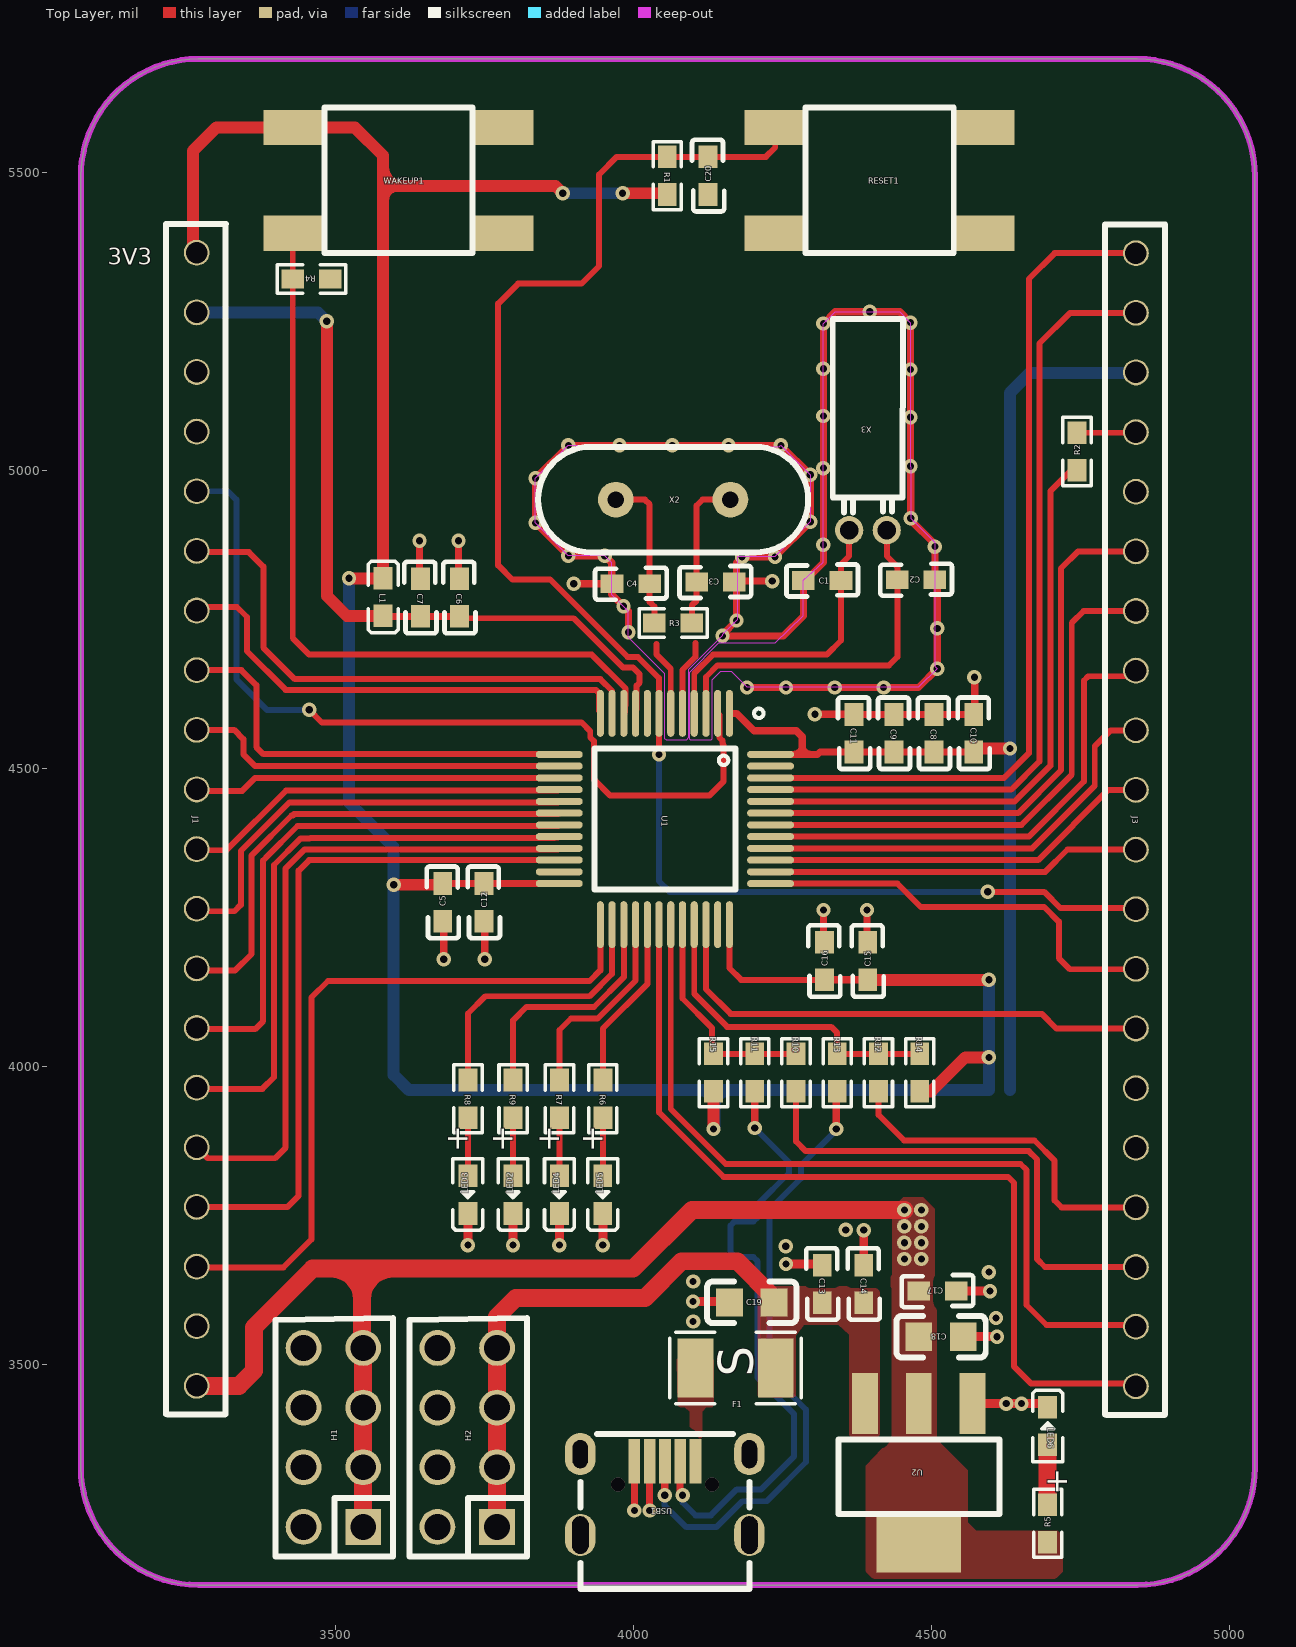
[diagram p0: Top Layer view]
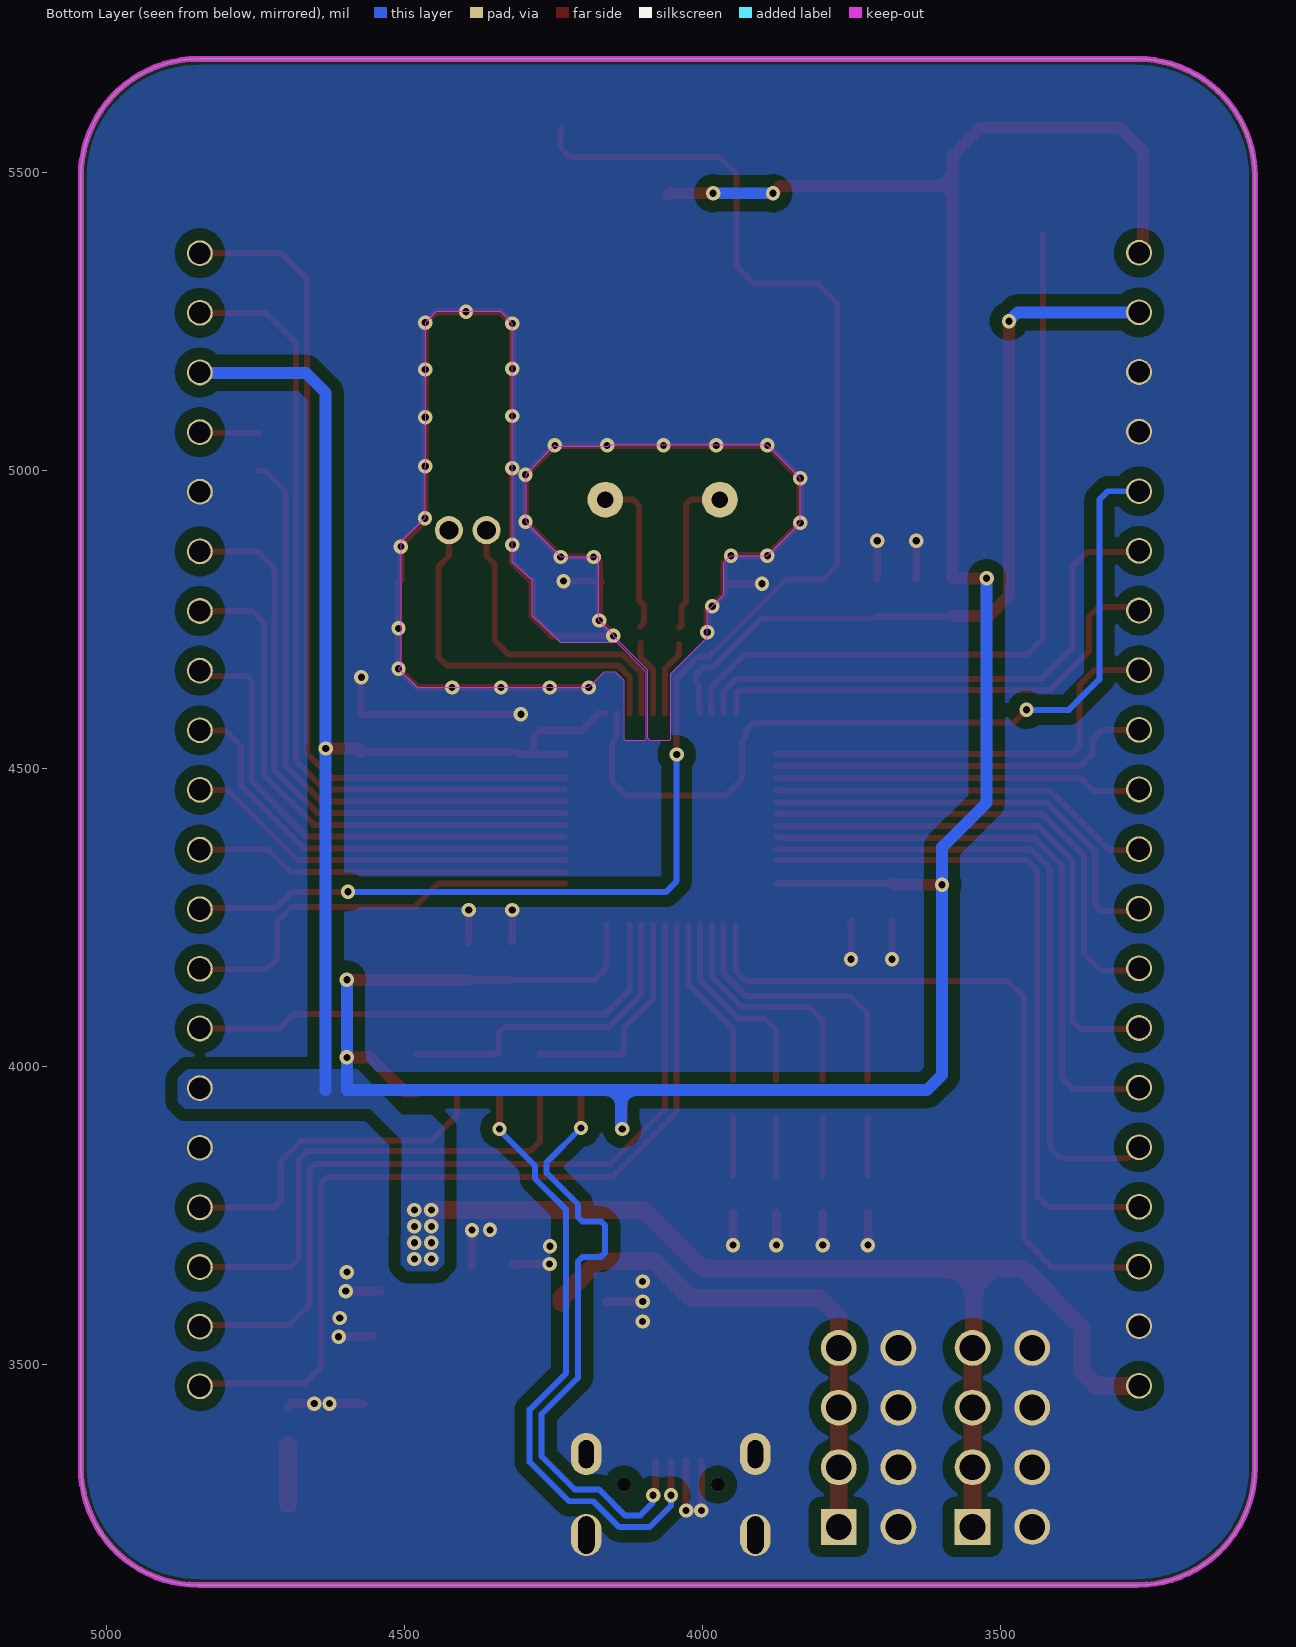
[diagram p1: Bottom Layer view, seen from below]
# Altium PCB MISC50188.pcbdoc
Units mil, origin at the board's own origin, x right, y up, seen from the top; angles counter-clockwise.
Board outline 1968.5 x 2559.06 mil, 2 copper layers (Top Layer, Bottom Layer), stack 62.206 mil thick; 53 components, 54 nets, 213 pads, 90 vias.

## Layer stack, top to bottom
Top Solder Mask Layer: solder mask 0.394, Dk 3.3
Top Layer: signal copper 1.379
Dielectric1: surface 59.449, FR4, Dk 4.5
Bottom Layer: signal copper 1.378
Bottom Solder Mask Layer: solder mask 0.394, Dk 3.3

## Board outline
3270.75,5689.88 ccw(c3270.75,5493.03) 3073.9,5493.03 3073.9,3327.68 ccw(c3270.75,3327.68) 3270.75,3130.83 4845.55,3130.83 ccw(c4845.55,3327.68) 5042.4,3327.68 5042.4,5493.03 ccw(c4845.55,5493.03) 4845.55,5689.88 3270.75,5689.88

## Design rules (kind name [scope] priority, off if disabled: settings)
BoardOutlineClearance copperThickness2oz_1 [All] p2 off: genericclearance=7.99 ignorepadtopadclearanceinfootprint=FALSE except(0: Arc-SplitContinuation Track-SplitContinuation SMDPad-SplitContinuation THPad-SplitContinuation Via-SplitContinuation Fill-SplitContinuation Region-SplitContinuation Poly-SplitContinuation Text-SplitContinuation Hole-SplitContinuation; 5.98: Arc-CutoutEdge Track-CutoutEdge SMDPad-CutoutEdge THPad-CutoutEdge Via-CutoutEdge Text-CutoutEdge; 6.9: Hole-OutlineEdge Hole-CutoutEdge; 11.81: Arc-OutlineEdge Track-OutlineEdge SMDPad-OutlineEdge THPad-OutlineEdge Via-OutlineEdge Fill-OutlineEdge Region-OutlineEdge Text-OutlineEdge Fill-CutoutEdge Region-CutoutEdge; 20: Poly-OutlineEdge Poly-CutoutEdge)
BoardOutlineClearance Plane_innerPlane_1 [All] p4 off: genericclearance=8 ignorepadtopadclearanceinfootprint=FALSE except(0: Arc-SplitContinuation Track-SplitContinuation SMDPad-SplitContinuation THPad-SplitContinuation Via-SplitContinuation Fill-SplitContinuation Region-SplitContinuation Poly-SplitContinuation Text-SplitContinuation Hole-SplitContinuation; 5.98: Arc-CutoutEdge Track-CutoutEdge SMDPad-CutoutEdge THPad-CutoutEdge Via-CutoutEdge Text-CutoutEdge; 6.9: Hole-OutlineEdge Hole-CutoutEdge; 10: Poly-OutlineEdge Poly-CutoutEdge; 11.81: Arc-OutlineEdge Track-OutlineEdge SMDPad-OutlineEdge THPad-OutlineEdge Via-OutlineEdge Fill-OutlineEdge Region-OutlineEdge Text-OutlineEdge Fill-CutoutEdge Region-CutoutEdge)
BoardOutlineClearance Copper_copperRegion_1 [All] p6 off: genericclearance=8 ignorepadtopadclearanceinfootprint=FALSE except(0: Arc-SplitContinuation Track-SplitContinuation SMDPad-SplitContinuation THPad-SplitContinuation Via-SplitContinuation Fill-SplitContinuation Region-SplitContinuation Poly-SplitContinuation Text-SplitContinuation Hole-SplitContinuation; 5.98: Arc-CutoutEdge Track-CutoutEdge SMDPad-CutoutEdge THPad-CutoutEdge Via-CutoutEdge Text-CutoutEdge; 6.9: Hole-OutlineEdge Hole-CutoutEdge; 10: Poly-OutlineEdge Poly-CutoutEdge; 11.81: Arc-OutlineEdge Track-OutlineEdge SMDPad-OutlineEdge THPad-OutlineEdge Via-OutlineEdge Fill-OutlineEdge Region-OutlineEdge Text-OutlineEdge Fill-CutoutEdge Region-CutoutEdge)
BoardOutlineClearance copperThickness1oz_1 [All] p8: genericclearance=8 ignorepadtopadclearanceinfootprint=FALSE except(0: Arc-SplitContinuation Track-SplitContinuation SMDPad-SplitContinuation THPad-SplitContinuation Via-SplitContinuation Fill-SplitContinuation Region-SplitContinuation Poly-SplitContinuation Text-SplitContinuation Hole-SplitContinuation; 5.98: Arc-CutoutEdge Track-CutoutEdge SMDPad-CutoutEdge THPad-CutoutEdge Via-CutoutEdge Text-CutoutEdge; 6.9: Hole-OutlineEdge Hole-CutoutEdge; 11.81: Arc-OutlineEdge Track-OutlineEdge SMDPad-OutlineEdge THPad-OutlineEdge Via-OutlineEdge Fill-OutlineEdge Region-OutlineEdge Text-OutlineEdge Fill-CutoutEdge Region-CutoutEdge; 20: Poly-OutlineEdge Poly-CutoutEdge)
Clearance copperThickness2oz [All] p1 off: gap=7.99 ignorepadtopadclearanceinfootprint=FALSE except(5.98: SMDPad-Track SMDPad-SMDPad THPad-Track SMDPad-THPad THPad-THPad Track-Via SMDPad-Via THPad-Via Via-Via Fill-SMDPad Region-SMDPad Fill-THPad Region-THPad Fill-Via Region-Via Fill-Fill Fill-Region Region-Region Arc-Track Arc-SMDPad Arc-THPad Arc-Via Fill-Arc Region-Arc Arc-Arc Text-Track SMDPad-Text Text-THPad Text-Via Fill-Text Region-Text Arc-Text Text-Text; 6.9: Hole-Track Hole-SMDPad Hole-THPad Hole-Via Fill-Hole Region-Hole Hole-Arc Hole-Text; 11.81: Fill-Track Region-Track; 20: Poly-Track Poly-SMDPad Poly-THPad Poly-Via Poly-Fill Poly-Region Poly-Poly Poly-Arc Poly-Text Poly-Hole)
Clearance Plane_innerPlane [All] p3 off: gap=8 ignorepadtopadclearanceinfootprint=FALSE except(5.98: SMDPad-Track SMDPad-SMDPad THPad-Track SMDPad-THPad THPad-THPad Track-Via SMDPad-Via THPad-Via Via-Via Fill-SMDPad Region-SMDPad Fill-THPad Region-THPad Fill-Via Region-Via Fill-Fill Fill-Region Region-Region Arc-Track Arc-SMDPad Arc-THPad Arc-Via Fill-Arc Region-Arc Arc-Arc Text-Track SMDPad-Text Text-THPad Text-Via Fill-Text Region-Text Arc-Text Text-Text; 6.9: Hole-Track Hole-SMDPad Hole-THPad Hole-Via Fill-Hole Region-Hole Hole-Arc Hole-Text; 10: Poly-Track Poly-SMDPad Poly-THPad Poly-Via Poly-Fill Poly-Region Poly-Poly Poly-Arc Poly-Text Poly-Hole; 11.81: Fill-Track Region-Track)
Clearance Copper_copperRegion [All] p5 off: gap=8 ignorepadtopadclearanceinfootprint=FALSE except(5.98: SMDPad-Track SMDPad-SMDPad THPad-Track SMDPad-THPad THPad-THPad Track-Via SMDPad-Via THPad-Via Via-Via Fill-SMDPad Region-SMDPad Fill-THPad Region-THPad Fill-Via Region-Via Fill-Fill Fill-Region Region-Region Arc-Track Arc-SMDPad Arc-THPad Arc-Via Fill-Arc Region-Arc Arc-Arc Text-Track SMDPad-Text Text-THPad Text-Via Fill-Text Region-Text Arc-Text Text-Text; 6.9: Hole-Track Hole-SMDPad Hole-THPad Hole-Via Fill-Hole Region-Hole Hole-Arc Hole-Text; 11.81: Fill-Track Region-Track; 20: Poly-Track Poly-SMDPad Poly-THPad Poly-Via Poly-Fill Poly-Region Poly-Poly Poly-Arc Poly-Text Poly-Hole)
Clearance copperThickness1oz [All] p7: gap=8 ignorepadtopadclearanceinfootprint=FALSE except(5.98: SMDPad-Track SMDPad-SMDPad THPad-Track SMDPad-THPad THPad-THPad Track-Via SMDPad-Via THPad-Via Via-Via Fill-SMDPad Region-SMDPad Fill-THPad Region-THPad Fill-Via Region-Via Fill-Fill Fill-Region Region-Region Arc-Track Arc-SMDPad Arc-THPad Arc-Via Fill-Arc Region-Arc Arc-Arc Text-Track SMDPad-Text Text-THPad Text-Via Fill-Text Region-Text Arc-Text Text-Text; 6.9: Hole-Track Hole-SMDPad Hole-THPad Hole-Via Fill-Hole Region-Hole Hole-Arc Hole-Text; 11.81: Fill-Track Region-Track; 20: Poly-Track Poly-SMDPad Poly-THPad Poly-Via Poly-Fill Poly-Region Poly-Poly Poly-Arc Poly-Text Poly-Hole)
DiffPairsRouting differentialPair [All] p1: maxlimit=6 minlimit=6 mostfreqgap=6 toplayer_minwidth=5 toplayer_prefwidth=10 toplayer_maxwidth=100 toplayer_mingap=6 toplayer_prefgap=6 toplayer_maxgap=6 bottomlayer_minwidth=5 bottomlayer_prefwidth=10 bottomlayer_maxwidth=100 bottomlayer_mingap=6 bottomlayer_prefgap=6 bottomlayer_maxgap=6 maxuncoupledlength=10
HoleToHoleClearance otherClearance [All] p1: gap=11.81 allowstackedmicrovias=TRUE
Length netLength [All] p1: minlimit=0 maxlimit=0
PasteMaskExpansion pasteMaskExpansion [All] p1: expansion=0
PlaneConnect innerPlane [All] p1: planeconnectstyle=Relief reliefexpansion=20 reliefentries=4 reliefconductorwidth=10 reliefairgap=10
PolygonConnect copperRegion [All] p1: connectstyle=Direct reliefconductorwidth=10 reliefentries=4 polygonreliefangle="90 Angle" airgapwidth=10 via.connectstyle=Relief via.reliefconductorwidth=10 via.reliefentries=4 via.polygonreliefangle="90 Angle" via.airgapwidth=10
RoutingVias viaSize [All] p1: holewidth=12.01 width=24.02 viastyle="Through Hole" minholewidth=11.81 minwidth=19.68 maxholewidth=248.03 maxwidth=393.7
SolderMaskExpansion solderMaskExpansion [IsVia] p1: expansion=-1000 istentingtop=TRUE
SolderMaskExpansion solderMaskExpansion [All] p2: expansion=2 istentingtop=FALSE
Width copperThickness2oz_2 [All] p1 off: maxlimit=100 minlimit=8 preferedwidth=10
Width power [(InNet('GND') OR InNet('VCC_3V3') OR InNet('VDDA') OR InNet('VIN_5V'))] p2: maxlimit=100 minlimit=10 preferedwidth=30
Width copperThickness1oz_2 [All] p3: maxlimit=100 minlimit=5 preferedwidth=10

## Components (designator, comment, footprint, x,y, rotation, side; value= is the part's Value field where it differs from the comment)
C1 "20pF" C0603 4316.93,3045.28 r0 top
C2 "20pF" C0603 4474.41,6586.61 r180 top
C3 "20pF" C0603 4137.8,6582.68 r180 top
C4 "20pF" C0603 3996.06,3039.93 r0 top
C5 "1uF" C0603 5450.78,4275.59 r90 top
C6 "10nF" C0603 1938.58,4786.54 r270 top
C7 "1uF" C0603 1873.2,4786.54 r270 top
C8 "1uF" C0603 2734.25,4559.06 r270 top
C9 "10nF" C0603 2667.32,4559.06 r270 top
C10 "1uF" C0603 2801.18,4559.06 r270 top
C11 "10nF" C0603 2600.39,4559.06 r270 top
C12 "10nF" C0603 5519.68,4275.59 r90 top
C13 "1uF" C0603 2546.93,3635.83 r270 top
C14 "10nF" C0603 2616.61,3635.83 r270 top
C15 "1uF" C0603 6163.38,4177.17 r90 top
C16 "10nF" C0603 6090.55,4177.17 r90 top
C17 "100nf" C0603 4510.24,5393.7 r180 top
C18 "10uf" C0805 4516.14,3547.25 r180 top
C19 "22uF" C0805 4198.9,3604.88 r0 top
C20 "100nF" C0603 5895.66,5494.09 r90 top
F1 "" F1210 4171.65,3494.88 r0 top
H1 "" HDR-TH_8P-P2.54-V-M-R2-C4-S2.54 3547.24,3228.35 r90 top
H2 "" HDR-TH_8P-P2.54-V-M-R2-C4-S2.54 3771.65,3228.35 r90 top
J1 "" HDR-TH_20PIN-V-MALE-PITCH2.54 3268.11,5364.88 r270 top
J3 "" HDR-TH_20PIN-V-MALE-PITCH2.54 4842.91,5364.09 r270 top
L1 "3.3uH" L0603 3580.71,4787.53 r270 top
LED2 "" LED0603 3798.42,3785.44 r90 top
LED3 "" LED0603 3722.83,3785.44 r90 top
LED4 "" LED0603 3876.27,3785.44 r90 top
LED5 "" LED0603 3949,3785.44 r90 top
LED6 "" LED0603 4694.88,3397.64 r270 top
R1 "10K" R0603 4057.08,5494.09 r270 top
R2 "10K" R0603 4744.09,5031.5 r90 top
R3 "1M" R0603 4066.93,4744.1 r0 top
R4 "10K" R0603 3460.63,5320.87 r180 top
R5 "1K" R0603 4694.88,3234.25 r90 top
R6 "1K" R0603 3949.2,3946.09 r270 top
R7 "1K" R0603 3876.47,3946.09 r270 top
R8 "1K" R0603 3723.03,3946.09 r270 top
R9 "1K" R0603 3798.62,3946.09 r270 top
R10 "0R" R0603 4272.94,3990.16 r270 top
R11 "NC/22R" R0603 4203.81,3990.16 r270 top
R12 "0R" R0603 4411.19,3990.16 r270 top
R13 "NC/22R" R0603 4342.06,3990.16 r270 top
R14 "NC/1.5K" R0603 4480.31,3990.16 r270 top
R15 "NC/1.5K" R0603 4134.69,3990.16 r270 top
RESET1 "" SW-SMD-T6X6-9.5X5.8 4413.38,5486.22 r0 top
U1 "" TQFP-48_L7.0-W7.0-P0.50-LS9.0-BL 4053.15,4415.35 r180 top
U2 "" SOT-223 4568.9,3435.04 r180 top
USB1 "" U-F-M5DD-Y-1 4053.15,3214.57 r180 top
WAKEUP1 "" SW-SMD-T6X6-9.5X5.8 3606.3,5486.22 r0 top
X2 "8MHz" OSC-49S-1 4066.93,4950.79 r0 top
X3 "32.768kHz" DT-38_BD3.1-P0.80 4393.7,4899.61 r180 top

## Footprints (in the part's own frame and the unit in brackets; to place one, negate y for a bottom-side part, rotate by r counter-clockwise, add the part's x,y. Pads: shape width x height; smd on the part's side, far side on the other; paste and mask are expansions set on the pad)
C0603 [mm]
  rect 0.965x0.8 smd: 1(-0.8,44.958) 2(0.8,44.958)
  silkscreen extent -1.52,44.27 1.52,45.64
C0805 [mm]
  rect 1.14x1.2 smd: 1(-0.95,0) 2(0.95,0)
  silkscreen extent -1.91,-0.89 1.91,0.89
DT-38_BD3.1-P0.80 [mm]
  round 1.2 hole 0.8: 1(-0.8,0) 2(0.8,0)
  silkscreen extent -1.5,-9 1.5,-0.76
F1210 [mm]
  rect 1.52x2.5 smd: 1(-1.71,0) 2(1.71,0)
  silkscreen extent -2.79,-1.52 2.79,1.52
HDR-TH_8P-P2.54-V-M-R2-C4-S2.54 [mil]
  rect 60x60 hole 43.31: 1(0,0)
  round 60 hole 43.31: 2(0,100) 3(100,0) 4(100,100) 5(200,0) 6(200,100) 7(300,0) 8(300,100)
  silkscreen extent -50,-50 350,147
HDR-TH_20PIN-V-MALE-PITCH2.54 [mm]
  round 1.1 hole 0.914: 1(0,0) 2(2.54,0) 3(5.08,0) 4(7.62,0) 5(10.16,0) 6(12.7,0) 7(15.24,0) 8(17.78,0) 9(20.32,0) 10(22.86,0) 11(25.4,0) 12(27.94,0) 13(30.48,0) 14(33.02,0) 15(35.56,0) 16(38.1,0) 17(40.64,0) 18(43.18,0) 19(45.72,0) 20(48.26,0)
  silkscreen extent -1.23,-1.31 49.49,1.25
L0603 [mm]
  rect 0.965x0.8 smd: 1(-0.8,0) 2(0.8,0)
  silkscreen extent -1.52,-0.64 1.52,0.64
LED0603 [mm]
  rect 0.965x0.8 smd: 1(-0.8,0) 2(0.8,0)
  silkscreen extent -1.52,-0.64 1.52,0.64
OSC-49S-1 [mil]
  round 60 hole 27.56: 1(-96.06,0) 2(96.06,0)
  silkscreen extent -226,-89 226,89
R0603 [mm]
  rect 0.965x0.8 smd: 1(-0.8,0) 2(0.8,0)
  silkscreen extent -1.45,-0.6 1.45,0.6
SOT-223 [mm]
  rect 1.1x2.6 smd: 1(0,0) 2(2.29,0) 3(4.58,0)
  rect 3.6x2.4 smd: 4(2.29,6)
  silkscreen extent -1.14,1.52 5.71,4.7
SW-SMD-T6X6-9.5X5.8 [mm]
  rect 2.5x1.5 smd: 1(-4.5,2.25) 2(4.5,2.25) 3(-4.5,-2.25) 4(4.5,-2.25)
  silkscreen extent -3.15,-3.1 3.15,3.1
TQFP-48_L7.0-W7.0-P0.50-LS9.0-BL [mm]
  oval 0.3x2 smd: 1(-2.75,-4.5) 2(-2.25,-4.5) 3(-1.75,-4.5) 4(-1.25,-4.5) 5(-0.75,-4.5) 6(-0.25,-4.5) 7(0.25,-4.5) 8(0.75,-4.5) 9(1.25,-4.5) 10(1.75,-4.5) 11(2.25,-4.5) 12(2.75,-4.5) 25(2.75,4.5) 26(2.25,4.5) 27(1.75,4.5) 28(1.25,4.5) 29(0.75,4.5) 30(0.25,4.5) 31(-0.25,4.5) 32(-0.75,4.5) 33(-1.25,4.5) 34(-1.75,4.5) 35(-2.25,4.5) 36(-2.75,4.5)
  oval 2x0.3 smd: 13(4.5,-2.75) 14(4.5,-2.25) 15(4.5,-1.75) 16(4.5,-1.25) 17(4.5,-0.75) 18(4.5,-0.25) 19(4.5,0.25) 20(4.5,0.75) 21(4.5,1.25) 22(4.5,1.75) 23(4.5,2.25) 24(4.5,2.75) 37(-4.5,2.75) 38(-4.5,2.25) 39(-4.5,1.75) 40(-4.5,1.25) 41(-4.5,0.75) 42(-4.5,0.25) 43(-4.5,-0.25) 44(-4.5,-0.75) 45(-4.5,-1.25) 46(-4.5,-1.75) 47(-4.5,-2.25) 48(-4.5,-2.75)
  silkscreen extent -4.2,-4.7 3,3
U-F-M5DD-Y-1 [mm]
  rect 0.5x1.9 smd: 1(-1.3,-3.15) 2(-0.65,-3.15) 3(0,-3.15) 4(0.65,-3.15) 5(1.3,-3.15)
  oval 1.3x1.8 hole 0.65 slot 1.2 at 90 deg: 6(-3.6,-3.45) 7(3.6,-3.45)
  oval 1.3x1.8 hole 0.7 slot 1.6 at 90 deg: 8(3.6,0) 9(-3.6,0)
  silkscreen extent -3.6,-4.3 3.6,2.3

## Via types
v1: diameter 24.02, hole 12, Top Layer to Bottom Layer, 88 vias
v2: diameter 23.62, hole 23.6, Top Layer to Bottom Layer, 2 vias

## Nets (pads, with @x,y where several pads share a name; then routed paths per layer and width w, separated by ;. In a path a pad name is that pad's centre, name@x,y a point inside that pad or via, vN(x,y) a via of type N, cw(c..) or ccw(c..) an arc to the next point about the centre after c; other vN are vias at no path point)
$1N278: LED5.2 R6.2 | length 97.7
  Top Layer w10: LED5.2 3949.2,3817.13 R6.2
$1N354: LED4.2 R7.2 | length 97.7
  Top Layer w10: LED4.2 3876.47,3817.13 R7.2
$1N427: LED3.2 R8.2 | length 97.7
  Top Layer w10: LED3.2 3723.03,3817.13 R8.2
$1N500: LED2.2 R9.2 | length 97.7
  Top Layer w10: LED2.2 3798.62,3817.13 R9.2
$1N3002: LED6.2 R5.2 | length 100.4
  Top Layer w30: R5.2 LED6.2
$1N3542: F1.1 USB1.1
$1N7842: J3.4 R2.2 | length 99.3
  Top Layer w10: R2.2 4841.81,5062.99 J3.4
$1N14164: R12.1 R13.1 R14.1 U1.33 | length 556.3
  Top Layer w10: U1.33 4102.36,4122.05 4157.48,4066.93 4332.06,4066.93 4342.06,4056.93 R13.1 R12.1 R14.1
$1N14239: R10.1 R11.1 R15.1 U1.32 | length 377.5
  Top Layer w10: U1.32 4082.68,4114.31 4131.89,4065.1 4131.89,4022.49 4132.72,4021.66 R15.1 R11.1 R10.1
BOOT0: R2.1 U1.44 | length 1013.5
  Top Layer w10: U1.44 4639.62,4444.88 4699.38,4504.64 4699.38,4965.14 4734.25,5000 R2.1
D+: R13.2 USB1.3 | length 1065.7
  Top Layer w12: v1(4052.86,3281.5) 4052.86,3338.3 USB1.3 ; v1(4340.55,3895.67) 4340.55,3957.15 R13.2
  Bottom Layer w10: v1(4052.86,3281.5) 4052.86,3263.99 4089,3227.86 4139.55,3227.86 4183.07,3271.37 4223.99,3271.37 4289.86,3337.25 4289.86,3424.99 4228.63,3486.22 4228.63,3759.93 4281.18,3812.48 4281.18,3834.34 4340.55,3893.7 v1(4340.55,3895.67)
D-: R11.2 USB1.2 | length 1065.3
  Top Layer w12: USB1.2 4078.74,3285.62 v1(4082.86,3281.5) ; v1(4203.81,3897.19) R11.2
  Bottom Layer w10: v1(4082.86,3281.5) 4082.77,3281.41 4082.77,3269.39 4104.42,3247.73 4130.22,3247.73 4173.74,3291.25 4214.66,3291.25 4269.99,3346.58 4269.99,3417.44 4208.75,3478.68 4208.75,3673.65 4201.68,3680.72 4170.45,3680.72 4163.38,3687.79 4163.38,3733.65 4170.45,3740.72 4201.68,3740.72 4208.75,3747.79 4208.75,3769.26 4261.31,3821.81 4261.31,3839.69 v1(4203.81,3897.19)
GND: C1.1 C2.1 C3.1 C4.1 C5.1 C6.1 C7.1 C8.1 C9.1 C10.1 C11.1 C12.1 C13.1 C14.1 C15.2 C16.2 C17.1 C18.1 C19.1 C20.1 H1.2 H1.4 H1.6 H1.8 H2.2 H2.4 H2.6 H2.8 J1.3 J1.4 J1.19 J3.5 J3.16 LED2.1 LED3.1 LED4.1 LED5.1 LED6.1 R4.1 RESET1.3 U1.8 U1.23 U1.35 U1.47 U2.1 USB1.4 USB1.5 USB1.6 USB1.7 USB1.8 USB1.9 | length 4596.1
  Top Layer w12: v1(3641.73,4881.89) 3641.73,4819.51 C7.1 ; C5.1 3682.26,4242.62 v1(3682.26,4180.25) ; v1(3707.11,4881.89) 3707.11,4819.51 C6.1 ; C12.1 3751.15,4242.62 v1(3751.15,4180.25) ; v1(3900.29,4809.9) 3962.66,4809.9 C4.1@3964.14,4811.38 ; v1(3992.12,4728.45) 3992.12,4763.78 v1(3983.83,4772.08) 3964.14,4791.77 C4.1@3964.14,4811.38 ; v1(4001.97,3255.91) USB1.5 ; v1(4027.56,3255.91) USB1.4 ; v1(4149.6,4722.44) 4251.97,4722.44 4285.43,4755.91 C1.1 4288.68,4815.28 4318.9,4845.5 v1(4318.9,4875.25) v1(4318.9,5003.71) v1(4318.9,5091.06) v1(4318.9,5170.19) v1(4318.9,5246.06) 4338.58,5265.75 v1(4396.62,5265.75) 4446.85,5265.75 v1(4464.94,5247.65) v1(4464.94,5169.12) v1(4464.9,5089) ; v1@4149.6,4724.41 v1(4173.23,4748.04) C3.1@4173.23,4814.15 ; C3.1 4170.77,4814.15 C3.1@4173.23,4814.15 ; v1(4190.94,4635.83) v1(4256.11,4635.83) v1(4337.97,4635.83) v1(4419.92,4635.83) 4478.34,4635.83 v1(4509.84,4667.32) v1(4509.84,4734.91) 4509.84,4812.68 C2.1 v1(4505.9,4872.05) ; v1(4233.14,4814.15) C3.1@4173.23,4814.15 ; v1(4304.58,4591.05) 4369.9,4591.05 C11.1 C9.1 C8.1 C10.1 ; v1(4319.07,4262.67) 4319.07,4210.14 C16.2 ; v1(4391.91,4262.67) 4391.91,4210.14 C15.2 ; v1(4464.9,5089) v1(4464.9,5006.79) 4465.45,5006.24 v1(4465.45,4919.5) ; v1@4465.45,4916.44 v1@4505.9,4875.99 ; C10.1@4571.18,4592.03 4572.64,4590.57 4572.64,4652.45 v1(4572.04,4653.05) ; C4.1@3964.14,4811.38 3964.14,4844.92 v1(3952.33,4856.73) v1(3891.3,4856.73) v1(3836.18,4911.85) v1(3836.18,4986.65) v1(3891.3,5041.77) v1(3977.03,5041.77) v1(4065.49,5041.77) v1(4159.94,5041.77) v1(4247.6,5041.77) v1(4296.81,4992.56) v1(4296.81,4913.82) v1(4237.76,4854.76) v1(4182.64,4854.76) 4173.23,4845.35 C3.1@4173.23,4814.15
  Top Layer w15: v1(3722.83,3700.79) LED3.1 ; v1(3798.42,3700.79) LED2.1 ; v1(3876.27,3700.79) LED4.1 ; v1(3949,3700.79) LED5.1 ; v1(4100.39,3606.3) 4160.07,3606.3 C19.1 ; v1(4256.37,3669.29) 4314.96,3669.29 C13.1 C13.1@4317.48,3667.87 ; v1(4386.61,3725.92) C14.1 C14.1@4387.16,3666.78 ; C17.1@4541.19,3623.15 C17.1 v1(4598.35,3623.7) ; C18.1 v1(4610.16,3547.25) ; U2.1 v1(4625.52,3435.04) v1(4651.16,3435.04) 4688.98,3435.04 LED6.1
  other v1: 4100.5,3572.83 4608.26,3578.74 4100.5,3639.88 4596.45,3655.52 4255.9,3698.82 4356.3,3726.38
NRST: C20.2 J3.12 R1.1 RESET1.1 U1.7 | length 2643.8
  Top Layer w10: v1(4043.3,4523.62) U1.7 4043.31,4651.57 4007.87,4687.01 3990.66,4687.01 3860.74,4816.93 3797.24,4816.93 3773.62,4840.55 3773.62,5279.53 3807.09,5312.99 3913.38,5312.99 3942.91,5342.52 3942.91,5496.06 3972.44,5525.59 R1.1 C20.2 4222.44,5525.59 4238.19,5541.34 4238.19,5572.83 RESET1.1 ; v1(4594.48,4293.31) 4688.97,4293.31 4716.53,4265.75 4841.26,4265.75 J3.12
  Bottom Layer w10: v1(4043.3,4523.62) 4043.3,4311.03 4061.02,4293.31 v1(4594.48,4293.31)
OSC32IN: C2.2 U1.3 X3.1 | length 615.7
  Top Layer w10: U1.3 4122.05,4653.55 4141.45,4672.95 4428.85,4672.95 4442.91,4687.01 C2.2 4442.91,4838.58 4425.19,4856.3 X3.1
OSC32OUT: C1.2 U1.4 X3.2 | length 526.6
  Top Layer w10: U1.4 4102.36,4659.45 4133.86,4690.95 4324.8,4690.95 4348.42,4714.57 C1.2 4348.42,4842.52 4362.2,4856.3 X3.2
OSC_IN: C3.2 R3.2 U1.5 X2.2 | length 396.3
  Top Layer w10: U1.5 4082.68,4665.36 4104.33,4687.01 4104.33,4710.63 ; R3.2@4104.33,4738.19 R3.2 4098.43,4773.63 4106.3,4781.5 C3.2 4106.3,4940.95 4116.14,4950.79 X2.2
OSC_OUT: C4.2 R3.1 U1.6 X2.1 | length 397.5
  Top Layer w10: X2.1 4019.68,4950.79 4027.56,4942.91 C4.2 4027.56,4779.53 4035.43,4771.65 R3.1 4035.43,4740.16 R3.1@4039.37,4736.22 ; 4039.37,4708.67 4039.37,4690.95 4062.99,4667.32 U1.6
PA0/WAKEUP: R4.2 U1.10 WAKEUP1.3 | length 1312.9
  Top Layer w10: WAKEUP1.3@3429.13,5395.67 R4.2 3429.13,4718.51 3456.69,4690.95 3930.49,4690.95 3987.05,4634.39 3987.05,4606 3985.94,4604.89 3985.94,4594.2 U1.10
PA1: J1.6 U1.11 | length 910.9
  Top Layer w10: J1.6 3270.08,4862.91 3355.59,4862.91 3379.92,4838.58 3379.92,4702.76 3432.79,4649.89 3944.86,4649.89 3964.57,4630.19 U1.11
PA2: J1.7 U1.12 | length 805.2
  Top Layer w10: J1.7 3274.02,4770.79 3335.51,4770.79 3352.36,4753.94 3352.36,4696.85 3417.32,4631.89 3937.41,4631.89 3942.91,4626.38 3942.91,4596.82 3944.34,4595.39 3944.34,4593.06 U1.12
PA3: J1.8 U1.13 | length 727.3
  Top Layer w10: J1.8 3342.99,4664.88 3368.11,4639.77 3368.11,4535.84 3379.92,4524.03 3875.58,4524.03 U1.13
PA4: J1.9 U1.14 | length 648.1
  Top Layer w10: J1.9 3330.79,4564.88 3346.46,4549.21 3346.46,4523.62 3366.14,4503.94 U1.14
PA5: J1.10 U1.15 | length 617.8
  Top Layer w10: J1.10 3270.39,4462.6 3344.49,4462.6 3366.14,4484.25 U1.15
PA6: J1.11 U1.16 | length 650.8
  Top Layer w10: J1.11 3270.08,4362.91 3317.9,4362.91 3417.87,4462.88 3874.3,4462.88 U1.16
PA7: J1.12 U1.17 | length 738.9
  Top Layer w10: J1.12 3270.08,4264.88 3274.31,4260.65 3331.51,4260.65 3342.24,4271.37 3342.24,4361.79 3423.36,4442.91 3868.24,4442.91 3868.53,4443.2 3874.3,4443.2 U1.17
PA8: R6.1 U1.29 | length 291.4
  Top Layer w10: R6.1 3949.2,4064.07 4023.62,4138.49 U1.29
PA9: J3.20 U1.30 | length 1485
  Top Layer w10: U1.30 4043.31,3923.36 4151.71,3814.96 4628.78,3814.96 4638.78,3804.96 4638.78,3497.05 4667.32,3468.51 4838.5,3468.51 J3.20
PA10: J3.19 U1.31 | length 1372.9
  Top Layer w10: U1.31 4062.99,3929.14 4155.23,3836.9 4649.45,3836.9 4659.45,3826.9 4659.45,3600.4 4692.91,3566.93 4840.07,3566.93 J3.19
PA11: J3.18 R10.2 | length 839.1
  Top Layer w10: R10.2 4272.94,3874.7 4289.37,3858.27 4663.53,3858.27 4677.45,3844.36 4677.45,3677.17 4690.52,3664.09 J3.18
PA12: J3.17 R12.2 | length 574.5
  Top Layer w10: R12.2 4411.41,3958.44 4411.41,3919.29 4454.44,3876.27 4672.94,3876.27 4706.69,3842.52 4706.69,3775.59 4718.19,3764.09 J3.17
PA15: J3.11 U1.38 | length 628.1
  Top Layer w10: U1.38 4690.94,4326.77 4728.26,4364.09 J3.11
PB0: J1.13 U1.18 | length 815.4
  Top Layer w10: J1.13 3271.57,4161.42 3332.68,4161.42 3360.24,4188.98 3360.24,4354.33 3427.16,4421.26 3429.27,4421.26 3431.52,4423.51 3874.3,4423.51 U1.18
PB1: J1.14 U1.19 | length 908.6
  Top Layer w10: J1.14 3270.08,4062.91 3366.06,4062.91 3379.64,4076.49 3379.64,4345.77 3383.86,4349.99 3383.86,4350.4 3437,4403.54 3868.24,4403.54 3868.53,4403.83 3874.3,4403.83 U1.19
PB2: J1.15 U1.20 | length 992.4
  Top Layer w10: J1.15 3270.08,3962.91 3378.26,3962.91 3397.64,3982.29 3397.64,4338.31 3441.78,4382.46 3457.39,4382.46 3458.79,4383.86 3868.24,4383.86 3868.53,4384.14 3874.3,4384.14 U1.20
PB3: J3.10 U1.39 | length 661.3
  Top Layer w10: U1.39 4679.13,4346.46 4796.77,4464.09 J3.10
PB4: J3.9 U1.40 | length 733.6
  Top Layer w10: U1.40 4669.15,4366.14 4773.9,4470.89 4773.9,4537.4 4800.59,4564.09 J3.9
PB5: J3.8 U1.41 | length 827
  Top Layer w10: U1.41 4663.38,4385.83 4755.9,4478.35 4755.9,4647.64 4762.97,4654.71 4833.53,4654.71 J3.8
PB6: J3.7 U1.42 | length 910.1
  Top Layer w10: U1.42 4651.16,4405.51 4735.38,4489.73 4735.38,4744.1 4755.38,4764.09 J3.7
PB7: J3.6 U1.43 | length 992.6
  Top Layer w10: U1.43 4645.39,4425.2 4717.38,4497.19 4717.38,4835.5 4745.98,4864.09 J3.6
PB8: J3.2 U1.45 | length 1354.3
  Top Layer w10: U1.45 4633.85,4464.57 4681.38,4512.1 4681.38,5212.88 4732.59,5264.09 J3.2
PB9: J3.1 U1.46 | length 1442.9
  Top Layer w10: U1.46 4622.04,4484.25 4663.38,4525.59 4663.38,5320.87 4706.61,5364.09 J3.1
PB10: J1.16 U1.21 | length 1105.1
  Top Layer w10: J1.16 3286.53,3846.46 3399.61,3846.46 3417.32,3864.18 3417.32,4332.54 3449.24,4364.46 3874.3,4364.46 U1.21
PB11: J1.17 U1.22 | length 1168.4
  Top Layer w10: J1.17 3297.64,3764.88 3297.93,3764.59 3420.09,3764.59 3438.98,3783.47 3438.98,4328.74 3456.69,4346.46 U1.22
PB12: J1.18 U1.25 | length 1197.9
  Top Layer w10: J1.18 3269.6,3663.39 3413.39,3663.39 3460.63,3710.63 3460.63,4116.14 3488.19,4143.7 3927.01,4143.7 3944.88,4161.58 U1.25
PB13: R8.1 U1.26 | length 463.1
  Top Layer w10: R8.1 3723.03,4089.18 3751.97,4118.11 3926.87,4118.11 3964.57,4155.81 U1.26
PB14: R9.1 U1.27 | length 404
  Top Layer w10: R9.1 3798.62,4077.87 3820.86,4100.11 3934.33,4100.11 3984.25,4150.04 U1.27
PB15: R7.1 U1.28 | length 339.6
  Top Layer w10: R7.1 3876.47,4061.51 3895.67,4080.71 3940.38,4080.71 4003.94,4144.26 U1.28
PC13/TAMPER_RTC: J1.5 U1.2 | length 1442.6
  Top Layer w10: v1(3456.69,4598.43) 3477.98,4577.14 3913.52,4577.14 3927.99,4562.66 3927.99,4552.06 3934.21,4545.84 3934.21,4481.77 3960.89,4455.09 4128.11,4455.09 4151.57,4478.55 4151.57,4539.73 4149.61,4541.7 4149.61,4546.98 4144.53,4552.06 4144.53,4589.72 U1.2
  Bottom Layer w10: J1.5 3320.55,4964.88 3334.64,4950.79 3334.64,4649.61 3385.83,4598.43 v1(3456.69,4598.43)
SWCLK: J3.13 U1.37 | length 707.2
  Top Layer w10: U1.37 4442.91,4307.09 4482.28,4267.72 4689.11,4267.72 4713.65,4243.18 4713.65,4182.02 4732.28,4163.39 J3.13@4842.21,4163.39
SWDIO: J3.14 U1.34 | length 856.4
  Top Layer w10: U1.34 4122.05,4129.92 4163.38,4088.59 4685.04,4088.59 4709.53,4064.09 J3.14
VCC_3V3: C5.2 C8.2 C9.2 C10.2 C11.2 C12.2 C15.1 C16.1 C17.2 C18.2 H1.1 H1.3 H1.5 H1.7 J1.1 J1.20 J3.3 J3.15 L1.1 R1.2 R5.1 R14.2 R15.2 U1.1 U1.24 U1.36 U1.48 U2.2 U2.4 WAKEUP1.1 | length 9029.5
  Top Layer w10: U1.36 4161.42,4165.36 4181.1,4145.67 C16.1
  Top Layer w12: C5.2 C12.2 U1.24 ; U1.1@4163.32,4592.52 4173.23,4592.52 4202.41,4563.33 4273.28,4563.33 4283.46,4553.15 4283.46,4537.61 ; U1.48 U1.48@4269.47,4523.62 ; 4283.46,4527.28 4283.46,4537.61 ; C16.1 C15.1 ; C10.2 C8.2 C9.2 C11.2 4312.99,4527.56 4309.05,4523.62 4297.45,4523.62 ; U1.48@4269.47,4523.62 4297.45,4523.62 ; U1.48@4269.47,4523.62 ccw(c4269.47,4537.61) 4283.46,4537.61 ; 4283.46,4537.61 ccw(c4297.45,4537.61) 4297.45,4523.62
  Top Layer w20: J1.1 3261.81,5371.18 3261.81,5535.43 3301.18,5574.8 WAKEUP1.1 3533.46,5574.8 3580.71,5527.56 3580.71,5507.73 ; v1(3523.62,4818.9) 3580.58,4818.9 L1.1 3580.71,5453.3 ; v1(3598.42,4305.12) 3678.81,4305.12 C5.2 ; v1(3881.89,5464.57) 3869.5,5476.96 3611.48,5476.96 ; v1(3982.28,5464.57) 4055.12,5464.57 R1.2 ; v1(4134.69,3895.67) R15.2 ; C15.1 v1(4596.45,4145.67) ; R14.2 4500,3958.66 4556.98,4015.65 v1(4596.45,4015.65) ; C10.2 4577.09,4533.47 v1(4631.89,4533.47) ; 3580.71,5453.3 3580.71,5507.73 ; 3580.71,5453.3 cw(c3604.37,5453.3) 3604.37,5476.96 3611.48,5476.96 ; 3580.71,5507.73 ccw(c3611.48,5507.73) 3611.48,5476.96
  Top Layer w30: J1.20 3338.89,3464.88 3364.17,3490.16 3364.17,3563 3462.6,3661.42 3493.41,3661.42 ; H1.1 H1.3 H1.5 H1.7 3545.27,3530.32 3545.27,3609.56 ; v1(4454.72,3759.85) 4098.42,3759.85 4000,3661.42 3597.14,3661.42 ; 3493.41,3661.42 3545.5,3661.42 ; 3493.41,3661.42 cw(c3493.41,3609.56) 3545.27,3609.56 ; 3545.27,3609.56 3545.27,3661.2 3545.5,3661.42 ; 3545.27,3609.56 cw(c3597.14,3609.56) 3597.14,3661.42 ; 3545.5,3661.42 3597.14,3661.42
  Bottom Layer w20: v1(3523.62,4818.9) 3523.62,4442.92 3598.42,4368.11 v1(3598.42,4305.12) 3598.42,3986.22 3624.01,3960.63 4136.4,3960.63 ; v1(3881.89,5464.57) v1(3982.28,5464.57) ; 4108.72,3960.63 4111.55,3960.63 cw(c4111.55,3935.78) 4136.4,3935.78 ; v1(4134.69,3895.67) 4136.4,3897.39 4136.4,3960.63 ; 4135.82,3937.01 cw(c4159.45,3937.01) 4159.45,3960.63 4162.41,3960.63 ccw(c4162.41,3934.63) 4136.4,3934.63 ; 4193.74,3960.63 4136.4,3960.63 ; 4199.65,3960.63 4596.45,3960.63 v1(4596.45,4015.65) v1(4596.45,4145.67) ; 4631.89,3960.63 v1(4631.89,4533.47) 4631.89,5129.92 4665.35,5163.39 4842.21,5163.39 J3.3
  other v1: 4454.72,3677.44 4483.28,3677.44 4454.72,3704.73 4483.28,3704.73 4454.72,3732.29 4483.28,3732.29 4483.28,3759.85
VDDA: C6.2 C7.2 J1.2 L1.2 U1.9 | length 1332.3
  Top Layer w10: C6.2 3711.66,4751.97 3900.25,4751.97 3983.21,4669.01 3999.94,4669.01 4010.83,4658.12 4010.83,4643.96 4005.75,4638.88 4005.75,4599.25 4003.94,4597.44 U1.9
  Top Layer w12: L1.2 3581.69,4755.05 C7.2 C6.2
  Top Layer w20: v1(3486.28,5250) 3486.28,4789.43 3519.68,4756.03 L1.2
  Bottom Layer w20: J1.2 3471.4,5264.88 v1(3486.28,5250)
VIN_5V: C13.2 C14.2 C19.2 F1.2 H2.1 H2.3 H2.5 H2.7 U2.3 | length 888.3
  Top Layer w30: H2.1 H2.3 H2.5 H2.7 3771.65,3580.71 3803.15,3612.21 4019.68,3612.21 4081.18,3673.7 4174.72,3673.7 4236.3,3612.13 C19.2
pads on no net: RESET1.2 RESET1.4 WAKEUP1.2 WAKEUP1.4
copper on no net:
  other v2: 3974.41,3299.21 4131.89,3299.21

## Polygon pours and split planes (outlines as drawn)
$1N3542 on Top Layer (solid, remove dead copper, pour order 0): 4114.17,3301.19 4094.49,3301.19 4094.49,3421.26 4086.61,3429.14 4074.8,3429.14 4072.83,3511.72 4134.68,3511.72 4134.68,3428.67 4122.41,3428.67 4116.14,3421.26 4116.14,3303.15
VIN_5V on Top Layer (solid, remove dead copper, pour order 2): 4210.63,3490.16 4210.63,3486.22 4217.15,3486.22 4216.95,3488.19 4212.6,3488.19
VIN_5V on Top Layer (solid, remove dead copper, pour order 4): 4272.7,3445.82 4208.66,3445.82 4208.66,3622.12 4216.87,3631.89 4404.73,3631.89 4413.51,3623.11 4413.51,3383.96 4411.35,3378.98 4364.18,3378.98 4362.2,3382.99 4362.2,3550.41 4343.65,3567.05 4286.89,3567.05 4272.7,3548.55
VCC_3V3 on Top Layer (solid, remove dead copper, pour order 6): 4575.2,3222.04 4561.02,3236.23 4561.02,3323.29 4509.27,3375.04 4509.27,3649.42 4498.03,3659.45 4448.82,3659.45 4432.24,3650.17 4432.24,3375.04 4389.76,3330.71 4389.76,3153.55 4401.57,3141.74 4708.66,3141.74 4720.47,3153.08 4720.47,3213.99 4711.81,3222.04
VCC_3V3 on Top Layer (solid, remove dead copper, pour order 8): 4434.52,3639.77 4434.52,3763.26 4452.75,3781.5 4486.22,3781.5 4505.9,3761.81 4505.9,3624.02 4450.26,3624.02
VCC_3V3 on Bottom Layer (solid, remove dead copper, pour order 10): 4504.05,3919.41 4578.79,3996.01 4864.22,3996.01 4879.92,3980.32 4879.92,3940.95 4868.11,3929.14 4557.08,3929.14 4504.41,3876.47 4505.9,3667.33 4495.9,3657.32 4445.04,3657.32 4433.07,3669.3 4433.07,3898.04 4454.44,3919.41
VCC_3V3 on Bottom Layer (solid, remove dead copper, pour order 12): 4548.68,3964.57 4549.21,3964.57 4549.44,3964.81
GND on Bottom Layer (solid, remove dead copper, pour order 14): 3000,5761.81 3000,3039.38 5220.47,3039.38 5220.47,5761.81

## Keep-outs
Board Outline Layer:
  region: 4096.45,4547.25 4094.49,4549.21 4094.49,4661.76 4143.36,4710.63 4238.19,4710.63 4285.43,4755.91 4285.43,4815.28 4318.9,4845.5 4318.9,5246.06 4338.58,5265.75 4446.85,5265.75 4464.94,5247.65 4464.94,5089.04 4464.9,5089 4464.9,5006.79 4465.45,5006.24 4465.45,4919.5 4505.9,4879.05 4505.9,4671.26 4509.84,4667.32 4478.34,4635.83 4190.94,4635.83 4164.88,4661.89 4146.14,4661.89 4131.89,4647.64 4131.89,4549.21 4129.92,4547.25
  region: 4053.15,4659.08 3992.12,4720.11 3992.12,4763.78 3964.14,4791.77 3964.14,4844.92 3952.33,4856.73 3891.3,4856.73 3836.18,4911.85 3836.18,4986.65 3891.3,5041.77 4157.05,5041.77 4159.45,5039.37 4245.2,5039.37 4247.6,5041.77 4296.81,4992.56 4296.81,4913.82 4237.76,4854.76 4174.77,4854.76 4174.77,4749.57 4149.6,4724.41 4149.6,4722.44 4092.52,4665.36 4092.52,4551.18 4088.58,4547.25 4055.92,4547.25 4053.15,4550.02
  lines w10: 3073.9,3327.68 3073.9,5493.03 cw(c3270.75,5493.03) 3270.75,5689.88 4845.55,5689.88 cw(c4845.55,5493.03) 5042.4,5493.03 5042.4,3327.68 cw(c4845.55,3327.68) 4845.55,3130.83 3270.75,3130.83 cw(c3270.75,3327.68) 3073.9,3327.68

## Silkscreen, mask and mechanical layers (free items; w line width, h text height)
Top Silkscreen Layer:
  text "3V3" at 3118.9,5344.88 h27.56